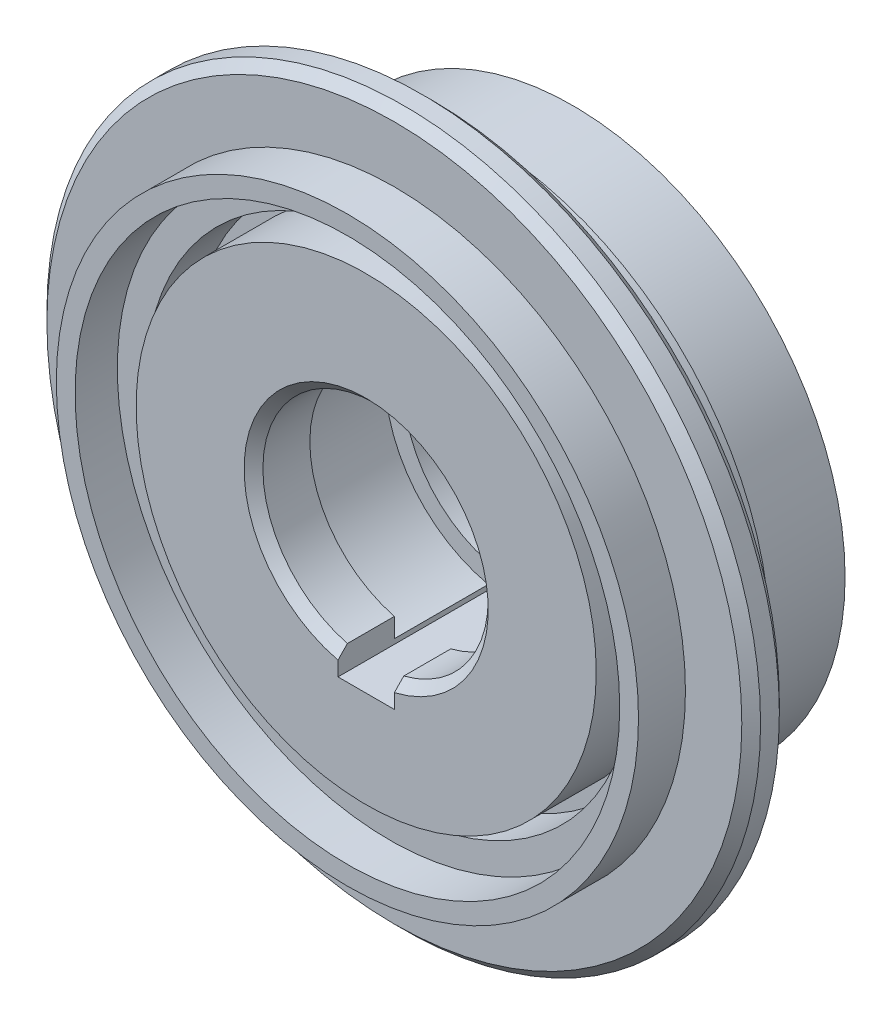
from build123d import *

# Parameters (mm, degrees)
CHAMFER_1_SIZE      = 1
SKETCH_3_W          = 6
SKETCH_3_H          = 4.4
CUT_EXTRUDE_1_DEPTH = 59.855755878
CHAMFER_2_SIZE      = 1


with BuildPart() as part:
    # 草图1 → 旋转1 (revolve)
    with BuildSketch(Plane(origin=(0, 0, 0), x_dir=(1, 0, 0), z_dir=(0, 1, 0)), mode=Mode.PRIVATE) as revolve_1_sk:
        Polygon((-12, 22), (-12, 16), (-14, 16), (-14, 6), (-12, 6), (-12, 0), (-24.5, 0), (-24.5, 7.5), (-29, 7.5), (-29, 22), align=None)
    revolve(revolve_1_sk.sketch.rotate(Axis((0, 0, 0), (0, 0, -1)), 180), axis=Axis((0, 0, 0), (0, 0, -1)))

    # 草图3 → 切除-拉伸1 (cut, through all)
    with BuildSketch(Plane(origin=(0, 0, -22), x_dir=(-1, 0, 0), z_dir=(0, 0, -1))):
        with Locations((0, -12)):
            Rectangle(SKETCH_3_W, SKETCH_3_H)
    extrude(amount=-CUT_EXTRUDE_1_DEPTH, mode=Mode.SUBTRACT)

    # 倒角2
    chamfer_2_edges = [part.edges().sort_by_distance(p)[0] for p in [
        (0, 12, 0),
        (0, 12, -22),
    ]]
    chamfer(chamfer_2_edges, length=CHAMFER_2_SIZE)


with BuildPart() as body_2:
    # 草图2 → 旋转2 (revolve)
    with BuildSketch(Plane(origin=(0, 0, 0), x_dir=(1, 0, 0), z_dir=(0, 1, 0)), mode=Mode.PRIVATE) as revolve_2_sk:
        Polygon((-29, 12), (-29, 7.5), (-26, 7.5), (-26, 2.5), (-29, 2.5), (-29, -2), (-31, -2), (-31, 3), (-38, 3), (-38, 7), (-31, 7), (-31, 12), align=None)
    revolve(revolve_2_sk.sketch.rotate(Axis((0, 0, 0), (0, 0, -1)), 180), axis=Axis((0, 0, 0), (0, 0, -1)))

    # 倒角1
    chamfer_1_edges = [body_2.edges().sort_by_distance(p)[0] for p in [
        (-38, 0, -7),
        (-38, 0, -3),
    ]]
    chamfer(chamfer_1_edges, length=CHAMFER_1_SIZE)


solid = Compound([part.part, body_2.part])
